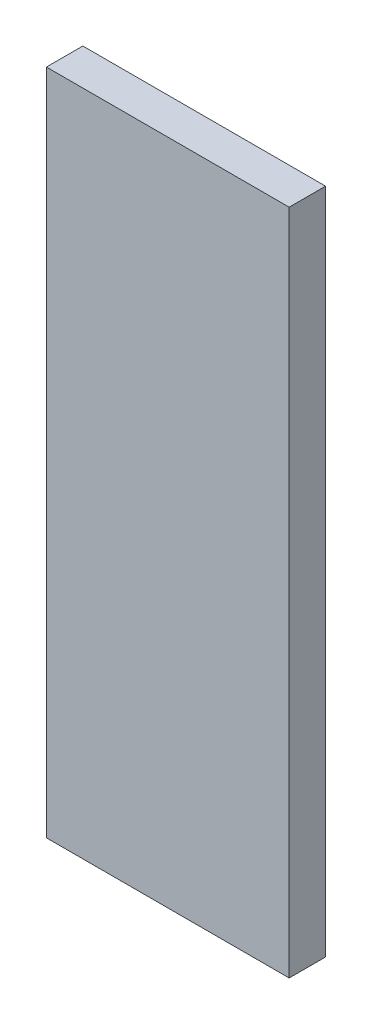
SolidWorks part; units mm, degrees
material "1023 carbon steel plate (SS)"
ref_plane "Front Plane" through (0, 0, 0) normal (0, 0, 1) x (1, 0, 0)
ref_plane "Top Plane" through (0, 0, 0) normal (0, 1, 0) x (1, 0, 0)
ref_plane "Right Plane" through (0, 0, 0) normal (1, 0, 0) x (0, 0, -1)
sketch "Sketch1" plane through (0, 0, 0) normal (0, 0, 1) x (1, 0, 0)
  line L1 (20, 55) -> (-20, 55)
  line L2 (20, 55) -> (20, -55)
  line L3 (20, -55) -> (-20, -55)
  line L4 (-20, 55) -> (-20, -55)
  line L5 (20, 55) -> (-20, -55) construction
  line L6 (20, -55) -> (-20, 55) construction
  point P0 (0, 0)
  dimension "D1" = 40
  dimension "D2" = 110
extrude "Boss-Extrude1" add sketch "Sketch1" along normal blind 6
